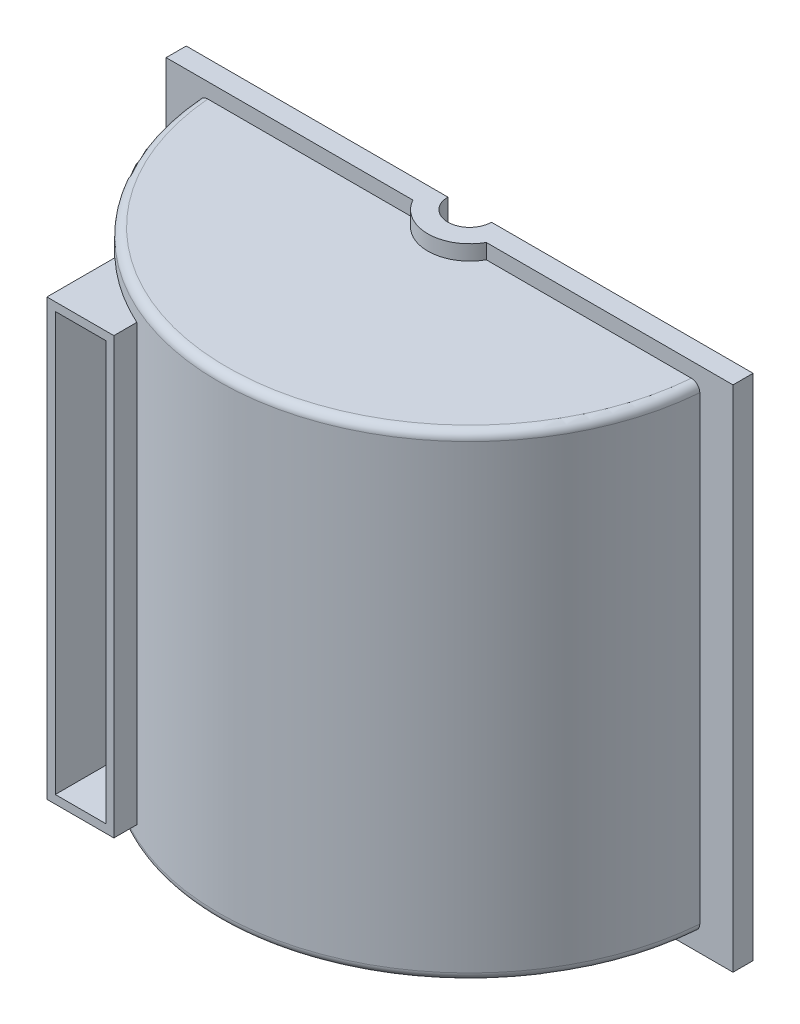
SolidWorks part; units mm, degrees
ref_plane "Front" through (0, 0, 0) normal (0, 0, 1) x (1, 0, 0)
ref_plane "Top" through (0, 0, 0) normal (0, 1, 0) x (1, 0, 0)
ref_plane "Right" through (0, 0, 0) normal (1, 0, 0) x (0, 0, -1)
sketch "Sketch1" plane through (0, 0, 0) normal (0, 1, 0) x (1, 0, 0)
  line L0 (-333.5, 0) -> (-333.5, -24)
  line L1 (-333.5, -24) -> (-298, -24)
  line L2 (-278, 0) -> (-333.5, 0)
  line L4 (-298, -24) -> (-298, -209.5799)
  line L5 (-333.5, -24) -> (-333.5, -228)
  line L6 (-333.5, -228) -> (-298, -228)
  line L7 (-298, -209.5799) -> (-333.5, -209.5799)
  line L8 (-333.5, -228) -> (-333.5, -209.5799)
  line L10 (-49.9092, -396.4688) -> (-60, -396.4688)
  line L11 (-60, -396.4688) -> (-60, -356.4688)
  line L12 (-60, -356.4688) -> (-298, -228)
  line L13 (-49.9092, -396.4688) -> (-49.9092, -352.3359)
  line L14 (-49.9092, -352.3359) -> (-285.1747, -220.7143)
  line L15 (-285.1747, -220.7143) -> (-286.793, -80.9554)
  line L16 (-49.9092, -273.4832) -> (-49.9092, -293.7909)
  arc A0 (-278, 0) -> (-49.9092, -273.4832) centre (0, 0) ccw
  arc A1 (-286.793, -80.9554) -> (-49.9092, -293.7909) centre (0, 0) ccw
  dimension "D1" = 556
  dimension "D2" = 596
  dimension "D3" = 333.5
  dimension "D5" = 24
  dimension "D8" = 40
extrude "Boss-Extrude1" add sketch "Sketch1" along normal mid plane 556 contours L15 A1 L16 A0 L2 L0 L1 L4 L7 L5 L6 L12 L11 L10 L13 L14
sketch "Sketch2" plane through (0, 278, 0) normal (0, 1, 0) x (1, 0, 0)
  line L0 (-278, 0) -> (-333.5, 0) construction
  line L1 (-298, 0) -> (5.2457, 0)
  line L2 (-298, 0) -> (-298, -209.3592)
  line L4 (5.2457, 0) -> (5.2457, -209.3592)
  line L5 (-298, -209.3592) -> (-298, -228)
  line L6 (-298, -228) -> (-60, -356.4688)
  line L7 (-60, -356.4688) -> (-60, -396.4688)
  line L8 (-60, -396.4688) -> (5.2457, -396.4688)
  line L9 (5.2457, -209.3592) -> (5.2457, -396.4688)
extrude "Boss-Extrude2" add sketch "Sketch2" against normal blind 10
mirror "Mirror2" about plane through (0, 0, 0) normal (0, 1, 0) of "Boss-Extrude2"
sketch "Sketch3" plane through (0, 278, 0) normal (0, 1, 0) x (1, 0, 0)
  line L0 (5.2457, 0) -> (5.2457, -50)
  line L1 (-333.5, -24) -> (-38.6177, -24)
  line L2 (-333.5, -24) -> (-333.5, 0)
  line L3 (-333.5, 0) -> (5.2457, 0)
  line L4 (5.2457, -24) -> (5.2457, 0)
  arc A0 (-38.6177, -24) -> (5.2457, -50) centre (5.2457, 0) ccw
  dimension "D1" = 100
extrude "Boss-Extrude3" add sketch "Sketch3" along normal blind 26 contours L0 A0 L1 L2 L3
mirror "Mirror3" about plane through (0, 0, 0) normal (0, 1, 0) of "Boss-Extrude3"
mirror "Mirror7" of "Mirror2", "Boss-Extrude2"
mirror "Mirror8" about plane through (5.2457, 268, 0) normal (1, 0, 0) of "Boss-Extrude1"
sketch "Sketch4" plane through (0, 278, 0) normal (0, 1, 0) x (1, 0, 0)
  line L0 (5.2457, -50) -> (5.2457, -24)
  line L1 (343.9914, -24) -> (49.1091, -24)
  line L2 (343.9914, -24) -> (343.9914, 0)
  line L3 (343.9914, 0) -> (5.2457, 0)
  line L4 (5.2457, -24) -> (5.2457, 0)
  arc A0 (5.2457, -50) -> (49.1091, -24) centre (5.2457, 0) ccw
extrude "Boss-Extrude4" add sketch "Sketch4" along normal blind 26
sketch "Sketch5" plane through (0, -278, 0) normal (0, -1, 0) x (1, 0, 0)
  line L0 (5.2457, 24) -> (5.2457, 50)
  line L1 (343.9914, 24) -> (49.1091, 24)
  line L2 (343.9914, 24) -> (343.9914, 0)
  line L3 (343.9914, 0) -> (5.2457, 0)
  line L4 (5.2457, 24) -> (5.2457, 0)
  arc A0 (49.1091, 24) -> (5.2457, 50) centre (5.2457, 0) ccw
extrude "Boss-Extrude5" add sketch "Sketch5" along normal blind 26
sketch "Sketch6" plane through (0, 304, 0) normal (0, 1, 0) x (1, 0, 0)
  line L0 (-333.5, 0) -> (343.9914, 0) construction
  circle A0 centre (5.2457, 0) radius 26
  dimension "D1" = 52
extrude "Cut-Extrude1" cut sketch "Sketch6" against normal through all
sketch "Sketch7" plane through (0, -278, 0) normal (0, -1, 0) x (1, 0, 0)
  line L0 (-38.6177, 24) -> (-390.2056, 24)
  line L1 (-390.2056, 24) -> (-390.2056, 451.7847)
  line L2 (-390.2056, 451.7847) -> (363.6416, 451.7847)
  line L3 (363.6416, 451.7847) -> (343.9914, 24)
  line L4 (343.9914, 24) -> (49.1091, 24)
  arc A0 (49.1091, 24) -> (-38.6177, 24) centre (5.2457, 0) ccw
extrude "Cut-Extrude2" cut sketch "Sketch7" against normal through all both and the other way through all
ref_plane "Plane1" through (0, -284, 0) normal (0, -1, 0) x (-1, 0, 0)
sketch "Sketch8" plane through (0, -284, 0) normal (0, -1, 0) x (-1, 0, 0)
  line L0 (294.7543, 0) -> (284.7543, 0)
  line L1 (-295.2457, 0) -> (-305.2457, 0)
  arc A0 (-305.2457, 0) -> (294.7543, 0) centre (-5.2457, 0) ccw
  arc A1 (-295.2457, 0) -> (284.7543, 0) centre (-5.2457, 0) ccw
  dimension "D1" = 600
  dimension "D2" = 580
extrude "Boss-Extrude6" add sketch "Sketch8" against normal blind 570
sketch "Sketch9" plane through (0, -284, 0) normal (0, -1, 0) x (1, 0, 0)
  line L0 (-38.6177, 24) -> (-293.7928, 24)
  line L1 (-283.7595, 24) -> (-293.7928, 24) construction
  line L2 (49.1091, 24) -> (304.2842, 24)
  line L3 (294.2509, 24) -> (304.2842, 24) construction
  arc A0 (304.2842, 24) -> (-293.7928, 24) centre (5.2457, 0) ccw
  arc A1 (49.1091, 24) -> (-38.6177, 24) centre (5.2457, 0) ccw
extrude "Boss-Extrude7" add sketch "Sketch9" against normal blind 10
sketch "Sketch10" plane through (0, 286, 0) normal (0, 1, 0) x (1, 0, 0)
  line L0 (-293.7928, -24) -> (-38.6177, -24)
  line L1 (304.2842, -24) -> (49.1091, -24)
  arc A0 (-38.6177, -24) -> (49.1091, -24) centre (5.2457, 0) ccw
  arc A1 (-293.7928, -24) -> (304.2842, -24) centre (5.2457, 0) ccw
extrude "Boss-Extrude8" add sketch "Sketch10" against normal blind 10
fillet "Fillet1" radius 10 2 edges at (5.2457, -284, 300) (5.2457, 286, 300)
ref_plane "Plane2" through (0, 0, 300) normal (0, 0, 1) x (1, 0, 0)
sketch "Sketch12" plane through (0, 0, 300) normal (0, 0, 1) x (1, 0, 0)
  line L1 (-200, 261) -> (-120, 261)
  line L2 (-200, 261) -> (-200, -259)
  line L3 (-200, -259) -> (-120, -259)
  line L4 (-120, 261) -> (-120, -259)
  line L5 (-38.6177, -304) -> (49.1091, -304) construction
  point P4 (-120, 1)
  dimension "D1" = 80
  dimension "D2" = 520
  dimension "D3" = 120
  dimension "D4" = 305
extrude "Boss-Extrude9" add sketch "Sketch12" against normal up to surface (27.3949 mm away)
sketch "Sketch13" plane through (0, 0, 300) normal (0, 0, 1) x (1, 0, 0)
  line L0 (-120, 261) -> (-200, 261) construction
  line L1 (-190, 251) -> (-129.462, 251)
  line L2 (-190, 251) -> (-190, -249)
  line L3 (-190, -249) -> (-129.462, -249)
  line L4 (-129.462, 251) -> (-129.462, -249)
  line L5 (-200, 261) -> (-200, -259) construction
  line L6 (-200, -259) -> (-120, -259) construction
  point P4 (-159.731, 251)
  point P7 (-160, 261)
  dimension "D1" = 10
  dimension "D2" = 10
  dimension "D3" = 10
extrude "Cut-Extrude3" cut sketch "Sketch13" against normal through all
